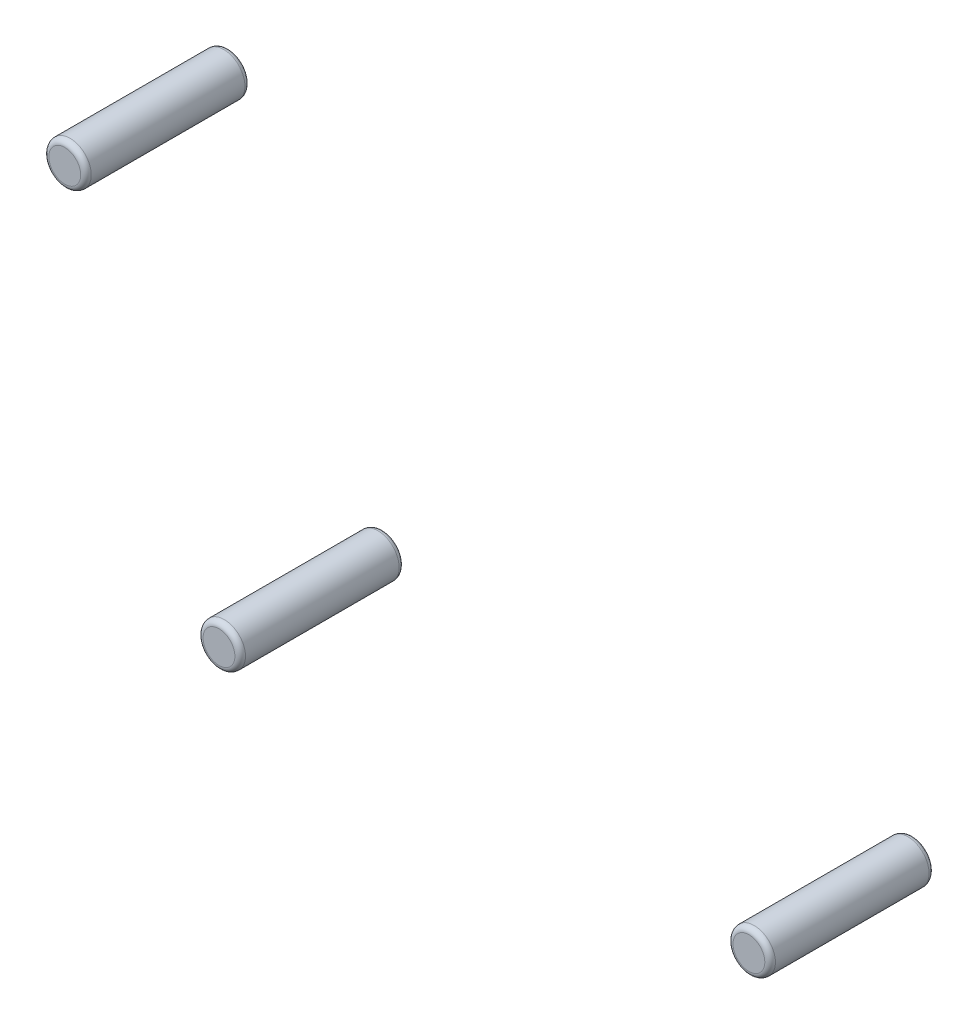
from build123d import *

# Parameters (mm, degrees)
BOSS_EXTRUDE1_DEPTH        = 26
BOSS_EXTRUDE1_DEPTH_BACK   = 5
SKETCH1_R                  = 4
BOSS_EXTRUDE1_2_DEPTH      = 26
BOSS_EXTRUDE1_2_DEPTH_BACK = 5
BOSS_EXTRUDE1_3_DEPTH      = 26
BOSS_EXTRUDE1_3_DEPTH_BACK = 5
FILLET1_R                  = 1
FILLET2_R                  = 1
FILLET3_R                  = 1


with BuildPart() as part:
    # Sketch1 → Boss-Extrude1 (new, two sides: drawn at the far end of the back side and taken through both)
    with BuildSketch(Plane.XY.offset(-BOSS_EXTRUDE1_DEPTH_BACK)):
        with Locations((-79.1, 0)):
            Circle(SKETCH1_R)
    extrude(amount=BOSS_EXTRUDE1_DEPTH + BOSS_EXTRUDE1_DEPTH_BACK)

    # Fillet1
    fillet1_edges = [part.edges().sort_by_distance(p)[0] for p in [
        (-83.1, 0, -5),
        (-83.1, 0, 26),
    ]]
    fillet(fillet1_edges, radius=FILLET1_R)


with BuildPart() as body_2:
    # Sketch1 → Boss-Extrude1 2 (new, two sides: drawn at the far end of the back side and taken through both)
    with BuildSketch(Plane.XY.offset(-BOSS_EXTRUDE1_2_DEPTH_BACK)):
        with Locations((-50, -64.1)):
            Circle(SKETCH1_R)
    extrude(amount=BOSS_EXTRUDE1_2_DEPTH + BOSS_EXTRUDE1_2_DEPTH_BACK)

    # Fillet2
    fillet2_edges = [body_2.edges().sort_by_distance(p)[0] for p in [
        (-54, -64.1, 26),
        (-54, -64.1, -5),
    ]]
    fillet(fillet2_edges, radius=FILLET2_R)


with BuildPart() as body_3:
    # Sketch1 → Boss-Extrude1 3 (new, two sides: drawn at the far end of the back side and taken through both)
    with BuildSketch(Plane.XY.offset(-BOSS_EXTRUDE1_3_DEPTH_BACK)):
        with Locations((50, -64.1)):
            Circle(SKETCH1_R)
    extrude(amount=BOSS_EXTRUDE1_3_DEPTH + BOSS_EXTRUDE1_3_DEPTH_BACK)

    # Fillet3
    fillet3_edges = [body_3.edges().sort_by_distance(p)[0] for p in [
        (46, -64.1, 26),
        (46, -64.1, -5),
    ]]
    fillet(fillet3_edges, radius=FILLET3_R)


solid = Compound([part.part, body_2.part, body_3.part])
